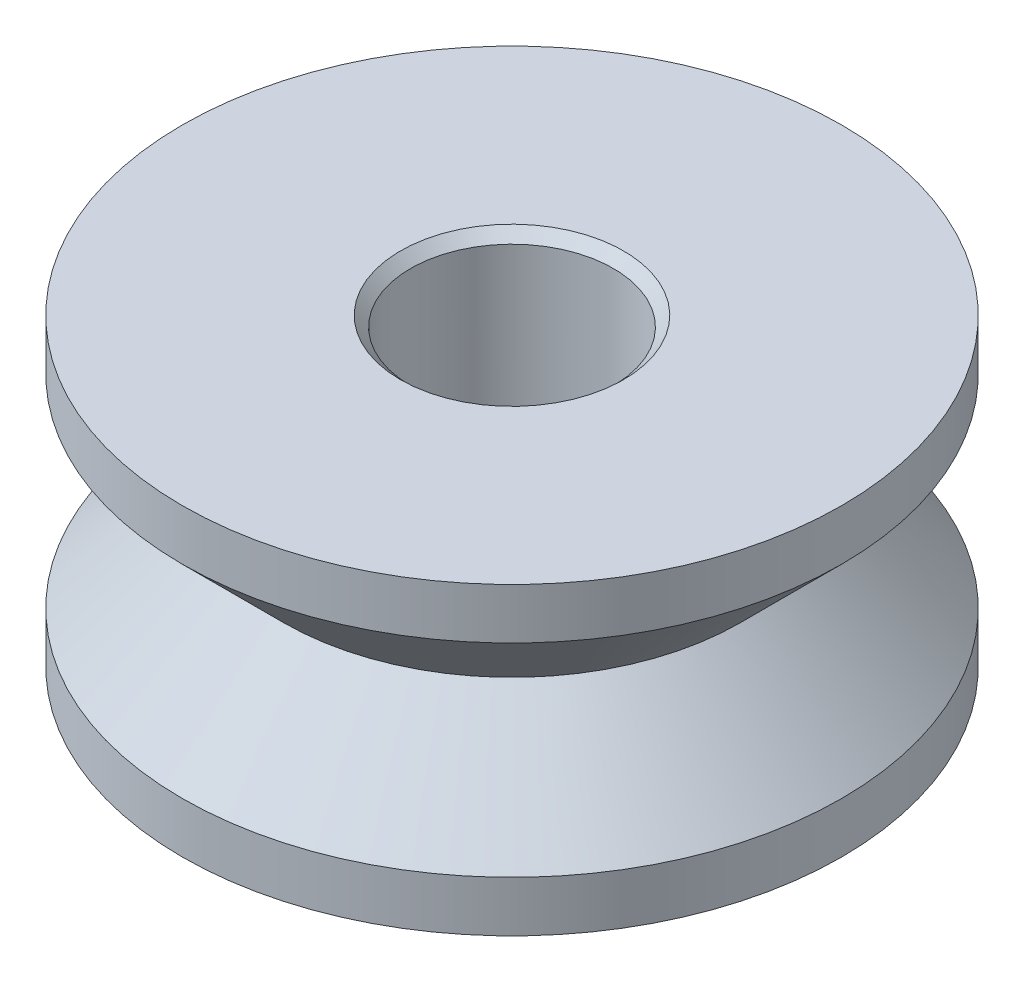
SolidWorks part; units mm, degrees
material "镀铬不锈钢"
ref_plane "前视基准面" through (0, 0, 0) normal (0, 0, 1) x (1, 0, 0)
ref_plane "上视基准面" through (0, 0, 0) normal (0, 1, 0) x (1, 0, 0)
ref_plane "右视基准面" through (0, 0, 0) normal (1, 0, 0) x (0, 0, -1)
ref_plane "基准面4" through (0, 2, 0) normal (0, 1, 0) x (1, 0, 0)
sketch "草图1" plane through (0, 0, 0) normal (0, 1, 0) x (1, 0, 0)
  circle A0 centre (0, 0) radius 4.5
  dimension "D1" = 9
sketch "草图2" plane through (0, 2, 0) normal (0, 1, 0) x (1, 0, 0)
  circle A0 centre (0, 0) radius 6.5
  dimension "D1" = 13
loft "放样1" add profiles "草图1", "草图2"
sketch "草图3" plane through (0, 2, 0) normal (0, 1, 0) x (1, 0, 0)
  circle A1 centre (0, 0) radius 6.5
  circle A2 centre (0, 0) radius 6.5
  dimension "D1" = 0
extrude "凸台-拉伸1" add sketch "草图3" along normal blind 1
mirror "镜向1" about plane through (0, 0, 0) normal (0, 1, 0) of "凸台-拉伸1", "放样1"
sketch "草图4" plane through (0, 3, 0) normal (0, 1, 0) x (1, 0, 0)
  circle A0 centre (0, 0) radius 2
  dimension "D1" = 4
extrude "切除-拉伸1" cut sketch "草图4" against normal through all
chamfer "倒角1" distance 0.2 angle 45 2 edges at (0, 3, 2) (0, -3, 2)
